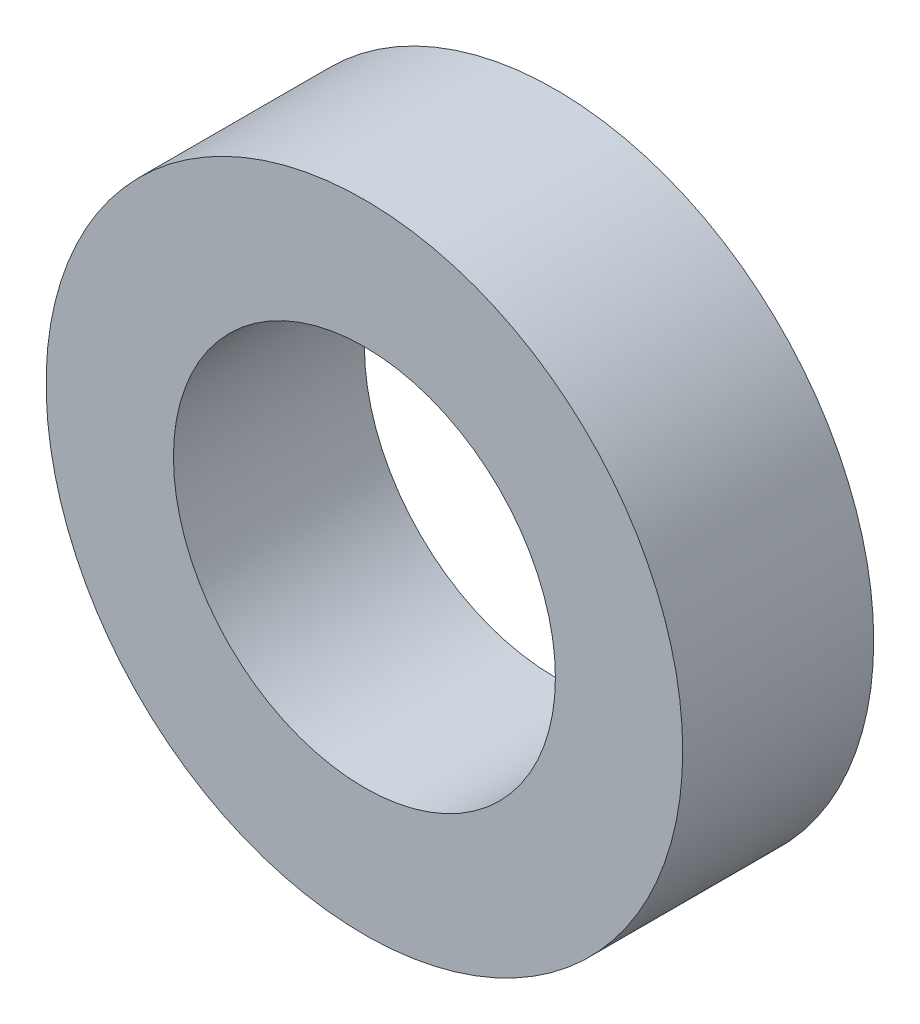
from build123d import *

# Parameters (mm, degrees)
SKETCH1_R           = 10
SKETCH1_R_2         = 6
BOSS_EXTRUDE1_DEPTH = 3


with BuildPart() as part:
    # Sketch1 → Boss-Extrude1 (new, symmetric)
    with BuildSketch(Plane.XY):
        Circle(SKETCH1_R)
        Circle(SKETCH1_R_2, mode=Mode.SUBTRACT)
    extrude(amount=BOSS_EXTRUDE1_DEPTH, both=True)


solid = part.part
